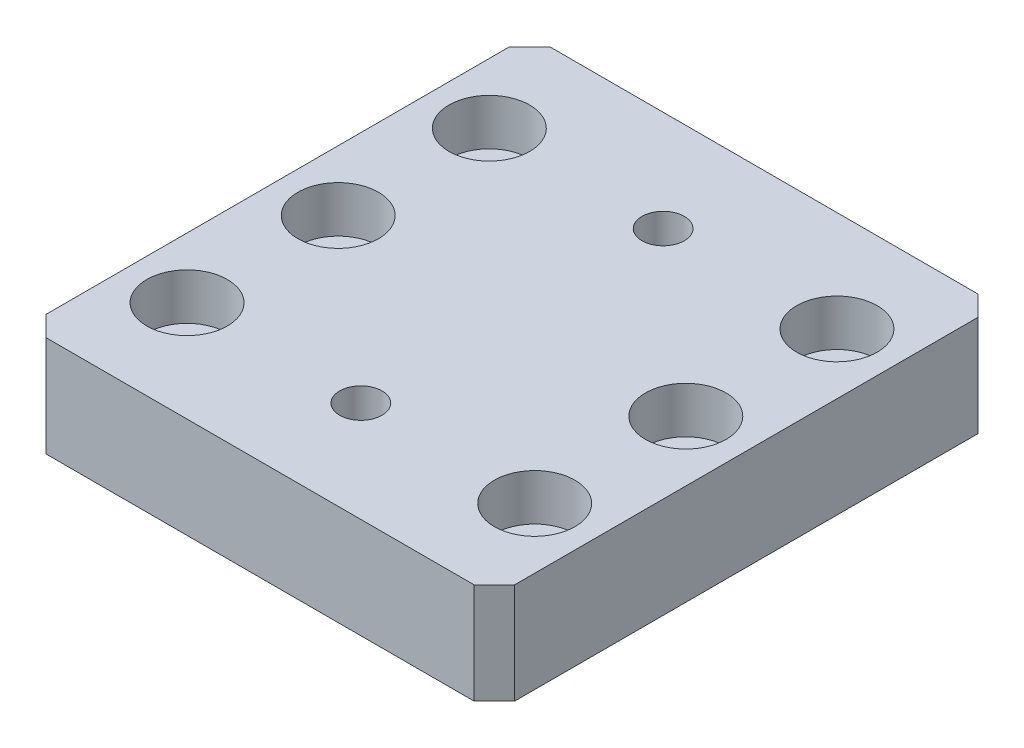
SolidWorks part; units mm, degrees
material "A6061 T6"
ref_plane "前视基准面" through (0, 0, 0) normal (0, 0, 1) x (1, 0, 0)
ref_plane "上视基准面" through (0, 0, 0) normal (0, 1, 0) x (1, 0, 0)
ref_plane "右视基准面" through (0, 0, 0) normal (1, 0, 0) x (0, 0, -1)
sketch "草图1" plane through (0, 0, 0) normal (0, 1, 0) x (1, 0, 0)
  line L1 (-23.25, 25) -> (23.25, 25)
  line L2 (-23.25, 25) -> (-23.25, -25)
  line L3 (-23.25, -25) -> (23.25, -25)
  line L4 (23.25, 25) -> (23.25, -25)
  line L5 (-23.25, 25) -> (23.25, -25) construction
  line L6 (-23.25, -25) -> (23.25, 25) construction
  point P0 (0, 0)
  dimension "D1" = 46.5
  dimension "D2" = 50
extrude "凸台-拉伸1" add sketch "草图1" along normal blind 10
hole_wizard "打孔尺寸(%根据)内六角圆柱头螺钉的类型1" positions "草图2" profile "草图3" counterbore size "M4" standard "GB"
sketch "草图2" plane through (0, 10, 0) normal (0, 1, 0) x (1, 0, 0)
  point P0 (17.25, -15)
  point P3 (17.25, 0)
  point P6 (17.25, 15)
  point P9 (-17.25, 15)
  point P12 (-17.25, 0)
  point P15 (-17.25, -15)
sketch "草图3" plane through (17.25, 10, 15) normal (1, 0, 0) x (0, 0, 1)
  line L0 (0, 0) -> (0, 21.3519)
  line L1 (0, 21.3519) -> (2.25, 20)
  line L2 (2.25, 20) -> (2.25, 4.6)
  line L3 (2.25, 4.6) -> (4, 4.6)
  line L4 (4, 4.6) -> (4, 0)
  line L5 (4, 0) -> (0, 0)
  line L10 (0, 21.3519) -> (-2.25, 20) construction
  line L11 (0, -6.35) -> (0, 107.95) construction
  dimension "孔直径" = 4.5
  dimension "孔深度" = 20
  dimension "柱形沉头孔直径" = 8
  dimension "柱形沉头孔深度" = 4.6
  dimension "导头角度" = 118
chamfer "倒角1" distance 2 angle 45 4 edges at (23.25, 5, 25) (-23.25, 5, 25) (-23.25, 5, -25) (23.25, 5, -25)
hole_wizard "M5 螺纹孔1" positions "草图4" profile "草图5" tap size "M5" standard "GB" end condition through all
sketch "草图4" plane through (0, 10, 0) normal (0, 1, 0) x (1, 0, 0)
  line L0 (21.25, 25) -> (-21.25, 25) construction
  line L1 (-21.25, -25) -> (21.25, -25) construction
  point P0 (0, 15)
  point P2 (0, -15)
  dimension "D1" = 10
  dimension "D2" = 10
sketch "草图5" plane through (0, 10, -15) normal (1, 0, 0) x (0, 0, 1)
  line L0 (0, 0) -> (0, 10)
  line L1 (0, 10) -> (2.1, 10)
  line L2 (2.1, 10) -> (2.1, 0)
  line L5 (2.1, 0) -> (0, 0)
  line L11 (0, -6.35) -> (0, 107.95) construction
  dimension "通孔螺纹孔钻头直径" = 4.2
  dimension "通孔螺纹孔钻头深度" = 10
cosmetic thread "孔螺蚊线1" parameters "D2"=5
cosmetic thread "孔螺蚊线2" parameters "D2"=5
